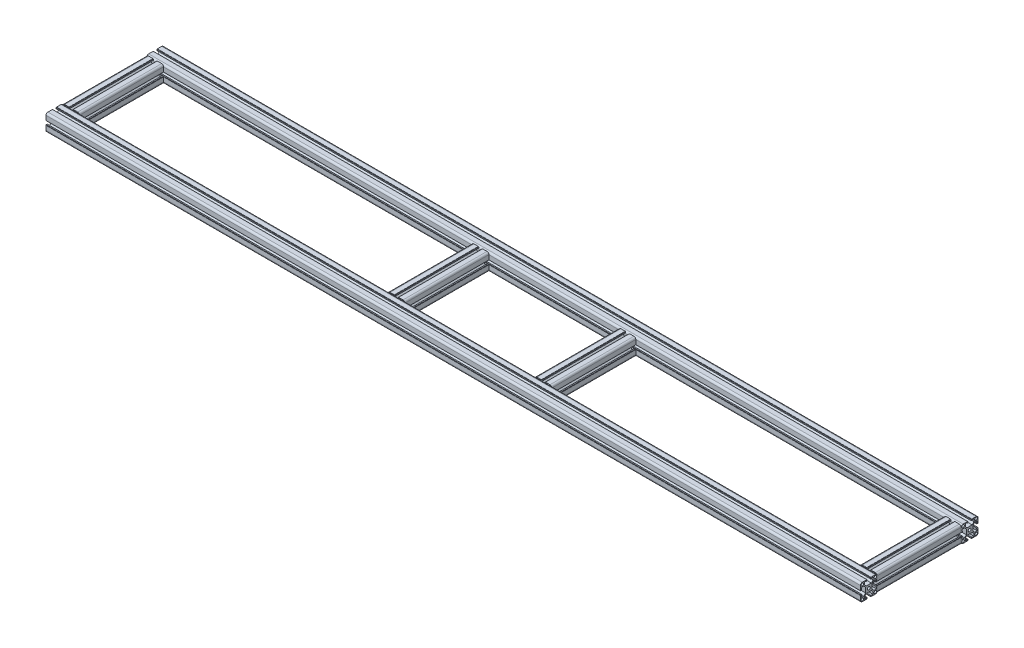
SolidWorks part; units mm, degrees
material "铝型材"
ref_plane "前基準面" through (0, 0, 0) normal (0, 0, 1) x (1, 0, 0)
ref_plane "上基準面" through (0, 0, 0) normal (0, 1, 0) x (1, 0, 0)
ref_plane "右基準面" through (0, 0, 0) normal (1, 0, 0) x (0, 0, -1)
sketch "草图1" plane through (0, 0, 0) normal (0, 1, 0) x (1, 0, 0)
  line L0 (-175, 120) -> (-175, -120)
  line L1 (-950, 120) -> (950, 120)
  line L2 (-950, 120) -> (-950, -120)
  line L3 (-950, -120) -> (950, -120)
  line L4 (950, 120) -> (950, -120)
  line L5 (0, 120) -> (0, -120) construction
  line L6 (175, 120) -> (175, -120)
  dimension "D1" = 1900
  dimension "D2" = 240
  dimension "D3" = 350
other "铝型材 40 X 40W X R4.5(1)"
ref_plane "基准面1" through (-950, 0, -120) normal (1, 0, 0) x (0, 0, -1)
sketch "Sketch1" plane through (-950, 0, -120) normal (1, 0, 0) x (0, 0, -1)
  line L0 (-5.1, 20) -> (-5.1, 19.5)
  line L1 (-5.1, 19.5) -> (-4.1, 19.5)
  line L2 (-4.1, 19.5) -> (-4.1, 17)
  line L3 (-6.1, 18) -> (-10.3, 18)
  line L4 (-15.5, -20) -> (-5.1, -20)
  line L5 (-20, -15.5) -> (-20, -5.1)
  line L6 (15.5, 20) -> (5.1, 20)
  line L7 (20, 15.5) -> (20, 5.1)
  line L8 (0, 20) -> (0, 0) construction
  line L9 (0, 0) -> (20, 0) construction
  line L10 (-10.3, 18) -> (-10.3, 12)
  line L11 (-10.3, 12) -> (-6, 7.7)
  line L12 (-6, 7.7) -> (6, 7.7)
  line L13 (10.3, 12) -> (6, 7.7)
  line L14 (10.3, 18) -> (10.3, 12)
  line L15 (6.1, 18) -> (10.3, 18)
  line L16 (4.1, 19.5) -> (4.1, 17)
  line L17 (5.1, 19.5) -> (4.1, 19.5)
  line L18 (5.1, 20) -> (5.1, 19.5)
  line L19 (-5.1, 20) -> (-15.5, 20)
  line L20 (20, 5.1) -> (19.5, 5.1)
  line L21 (0, 0) -> (-15.5563, 15.5563) construction
  line L22 (0, 0) -> (-15.5563, -15.5563) construction
  line L23 (0, 20) -> (0, 40) construction
  line L24 (20, 0) -> (40, 0) construction
  line L25 (19.5, 5.1) -> (19.5, 4.1)
  line L26 (19.5, 4.1) -> (17, 4.1)
  line L27 (17, 6.1) -> (17, 4.1)
  line L28 (18, 6.1) -> (17, 6.1)
  line L29 (18, 6.1) -> (18, 10.3)
  line L30 (18, 10.3) -> (12, 10.3)
  line L31 (12, 10.3) -> (7.7, 6)
  line L32 (7.7, 6) -> (7.7, -6)
  line L33 (12, -10.3) -> (7.7, -6)
  line L34 (18, -10.3) -> (12, -10.3)
  line L35 (18, -6.1) -> (18, -10.3)
  line L36 (18, -6.1) -> (17, -6.1)
  line L37 (17, -4.1) -> (17, -6.1)
  line L38 (19.5, -4.1) -> (17, -4.1)
  line L39 (19.5, -5.1) -> (19.5, -4.1)
  line L40 (20, -5.1) -> (19.5, -5.1)
  line L41 (5.1, -20) -> (5.1, -19.5)
  line L42 (5.1, -19.5) -> (4.1, -19.5)
  line L43 (4.1, -19.5) -> (4.1, -17)
  line L44 (6.1, -17) -> (4.1, -17)
  line L45 (6.1, -18) -> (6.1, -17)
  line L46 (6.1, -18) -> (10.3, -18)
  line L47 (10.3, -18) -> (10.3, -12)
  line L48 (10.3, -12) -> (6, -7.7)
  line L49 (6, -7.7) -> (-6, -7.7)
  line L50 (-10.3, -12) -> (-6, -7.7)
  line L51 (-10.3, -18) -> (-10.3, -12)
  line L52 (-6.1, -18) -> (-10.3, -18)
  line L53 (-6.1, -18) -> (-6.1, -17)
  line L54 (-4.1, -17) -> (-6.1, -17)
  line L55 (-4.1, -19.5) -> (-4.1, -17)
  line L56 (-5.1, -19.5) -> (-4.1, -19.5)
  line L57 (-5.1, -20) -> (-5.1, -19.5)
  line L58 (-20, -5.1) -> (-19.5, -5.1)
  line L59 (5.1, -20) -> (15.5, -20)
  line L60 (-20, 5.1) -> (-20, 15.5)
  line L61 (-19.5, -5.1) -> (-19.5, -4.1)
  line L62 (-6.1, 18) -> (-6.1, 17)
  line L63 (-6.1, 17) -> (-4.1, 17)
  line L64 (6.1, 18) -> (6.1, 17)
  line L65 (4.1, 17) -> (6.1, 17)
  line L66 (-19.5, -4.1) -> (-17, -4.1)
  line L71 (-17, -6.1) -> (-17, -4.1)
  line L72 (-18, -6.1) -> (-17, -6.1)
  line L73 (-18, -6.1) -> (-18, -10.3)
  line L74 (-18, -10.3) -> (-12, -10.3)
  line L75 (-12, -10.3) -> (-7.7, -6)
  line L76 (-7.7, -6) -> (-7.7, 6)
  line L77 (-12, 10.3) -> (-7.7, 6)
  line L78 (-18, 10.3) -> (-12, 10.3)
  line L79 (-18, 6.1) -> (-18, 10.3)
  line L80 (-18, 6.1) -> (-17, 6.1)
  line L81 (-17, 4.1) -> (-17, 6.1)
  line L82 (-19.5, 4.1) -> (-17, 4.1)
  line L83 (-19.5, 5.1) -> (-19.5, 4.1)
  line L84 (-20, 5.1) -> (-19.5, 5.1)
  line L85 (20, -5.1) -> (20, -15.5)
  circle A0 centre (0, 0) radius 3.4
  arc A1 (-20, 15.5) -> (-15.5, 20) centre (-15.5, 15.5) cw
  arc A2 (20, 15.5) -> (15.5, 20) centre (15.5, 15.5) ccw
  arc A3 (-15.5, -20) -> (-20, -15.5) centre (-15.5, -15.5) cw
  arc A4 (15.5, -20) -> (20, -15.5) centre (15.5, -15.5) ccw
  circle A5 centre (-15.5563, 15.5563) radius 3
  circle A6 centre (15.5563, 15.5563) radius 3
  circle A7 centre (15.5563, -15.5563) radius 3
  circle A8 centre (-15.5563, -15.5563) radius 3
  point P2 (0, 10)
  point P4 (0, 0)
  point P5 (-20, -20)
  point P6 (20, -20)
  point P7 (20, 20)
  point P8 (-20, 20)
  point P13 (20, 0)
  point P36 (-20, 20)
  point P39 (20, 20)
  point P43 (0, 20)
  point P50 (-40, 0)
  point P59 (0, 40)
  point P72 (40, 0)
  point P73 (-20, 0)
  point P86 (10, 0)
  point P87 (-10, 0)
  point P88 (0, -10)
  point P89 (0, -20)
  point P117 (0, -40)
  point P118 (0, 0)
  dimension "D1" = 20.6
  dimension "D2" = 40
  dimension "D3" = 8.2
  dimension "D4" = 10.2
  dimension "D5" = 12.3
  dimension "D6" = 6.8
  dimension "D7" = 4.5
  dimension "D8" = 45
  dimension "D12" = 6
  dimension "D13" = 22
  dimension "D9" = 0.5
  dimension "D10" = 2
  dimension "D11" = 12
  dimension "D16" = 3
  dimension "D17" = 2
